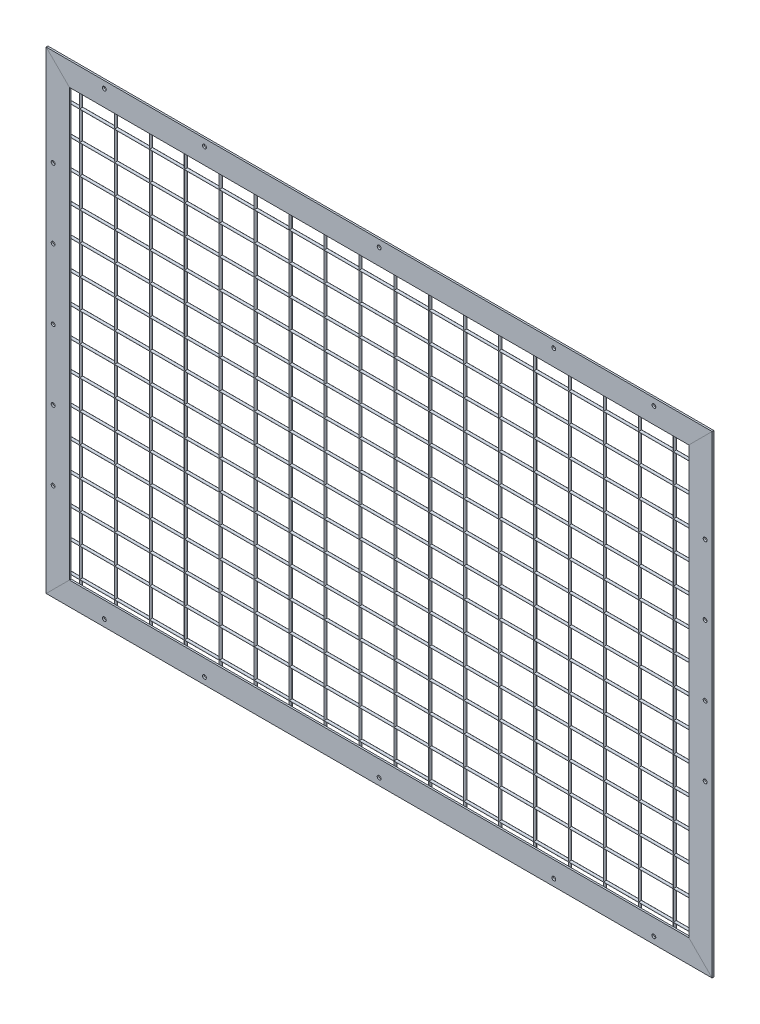
SolidWorks part; units mm, degrees
material "Q235-A GB/T700-2006"
material "Q235-A GB/T700-2006"
material "Q235-A GB/T700-2006"
material "Q235-A GB/T700-2006"
material "Q235-A GB/T700-2006"
material "Q235-A GB/T700-2006"
ref_plane "前视" through (0, 0, 0) normal (0, 0, 1) x (1, 0, 0)
ref_plane "上视" through (0, 0, 0) normal (0, 1, 0) x (1, 0, 0)
ref_plane "右视" through (0, 0, 0) normal (1, 0, 0) x (0, 0, -1)
sketch "草图4" plane through (0, 0, 0) normal (0, 0, 1) x (1, 0, 0)
  line L1 (0, 0) -> (40, 40)
  line L2 (0, 0) -> (0, 813)
  line L3 (0, 813) -> (40, 773)
  line L4 (40, 40) -> (40, 773)
  line L5 (1104, 40) -> (1144, 0)
  line L6 (1104, 40) -> (1104, 773)
  line L7 (1104, 773) -> (1144, 813)
  line L8 (1144, 0) -> (1144, 813)
  dimension "D1" = 813
  dimension "D2" = 45
  dimension "D3" = 1144
  dimension "D4" = 40
  dimension "D5" = 45
  dimension "D6" = 45
  dimension "D7" = 45
extrude "凸台-拉伸2" add sketch "草图4" along normal blind 3
sketch "草图6" plane through (0, 0, 3) normal (0, 0, 1) x (1, 0, 0)
  line L0 (1104, 773) -> (1104, 40) construction
  line L1 (0, 0) -> (1144, 0)
  line L2 (0, 0) -> (40, 40)
  line L3 (40, 40) -> (1104, 40)
  line L4 (1144, 0) -> (1104, 40)
  line L5 (40, 773) -> (0, 813) construction
  line L6 (0, 813) -> (1144, 813)
  line L7 (0, 813) -> (40, 773)
  line L8 (40, 773) -> (1104, 773)
  line L9 (1144, 813) -> (1104, 773)
  line L10 (1144, 0) -> (1144, 813) construction
  line L11 (1144, 813) -> (1104, 773) construction
  line L12 (0, 0) -> (40, 40) construction
extrude "凸台-拉伸3" add sketch "草图6" against normal up to surface (3 mm away) separate body up to face at (20, 406.5, 0)
ref_plane "基准面1" through (0, 25, 0) normal (0, -1, 0) x (-1, 0, 0)
ref_plane "基准面2" through (25, 0, 0) normal (-1, 0, 0) x (0, 0, 1)
sketch "草图7" plane through (0, 25, 0) normal (0, -1, 0) x (-1, 0, 0)
  line L0 (0, 0) -> (-1144, 0) construction
  line L1 (0, -3) -> (0, 0) construction
  circle A0 centre (-55, 2) radius 2
  circle A1 centre (-115, 2) radius 2
  circle A2 centre (-175, 2) radius 2
  circle A3 centre (-235, 2) radius 2
  circle A4 centre (-295, 2) radius 2
  circle A5 centre (-355, 2) radius 2
  circle A6 centre (-415, 2) radius 2
  circle A7 centre (-475, 2) radius 2
  circle A8 centre (-535, 2) radius 2
  circle A9 centre (-595, 2) radius 2
  circle A10 centre (-655, 2) radius 2
  circle A11 centre (-715, 2) radius 2
  circle A12 centre (-775, 2) radius 2
  circle A13 centre (-835, 2) radius 2
  circle A14 centre (-895, 2) radius 2
  circle A15 centre (-955, 2) radius 2
  circle A16 centre (-1015, 2) radius 2
  circle A17 centre (-1075, 2) radius 2
  circle A20 centre (-1195, 2) radius 2 [skipped]
  circle A21 centre (-1135, 2) radius 2 [skipped]
  dimension "D1" = 4
  dimension "D2" = 55
  dimension "D3" = 20
extrude "凸台-拉伸4" add sketch "草图7" against normal offset from surface (763 mm away) 25 separate body up to face at (572, 813, 1.5)
sketch "草图8" plane through (25, 0, 0) normal (-1, 0, 0) x (0, 0, 1)
  line L0 (0, 813) -> (0, 0) construction
  line L2 (-4, 25) -> (0, 25) construction
  circle A0 centre (-2, 47.1) radius 2
  circle A1 centre (-2, 97.1) radius 2
  circle A2 centre (-2, 147.1) radius 2
  circle A3 centre (-2, 197.1) radius 2
  circle A4 centre (-2, 247.1) radius 2
  circle A5 centre (-2, 297.1) radius 2
  circle A6 centre (-2, 347.1) radius 2
  circle A7 centre (-2, 397.1) radius 2
  circle A8 centre (-2, 447.1) radius 2
  circle A9 centre (-2, 497.1) radius 2
  circle A10 centre (-2, 547.1) radius 2
  circle A11 centre (-2, 597.1) radius 2
  circle A12 centre (-2, 647.1) radius 2
  circle A13 centre (-2, 697.1) radius 2
  circle A14 centre (-2, 747.1) radius 2
  dimension "D1" = 4
  dimension "D2" = 22.1
  dimension "D4" = 5
  dimension "D3" = 11
extrude "凸台-拉伸5" add sketch "草图8" against normal offset from surface (1094 mm away) 25 up to face at (1144, 406.5, 1.5)
hole_wizard "M6 间隙孔1" positions "草图10" profile "草图9" hole size "M6" standard "ISO" end condition up to next
sketch "草图10" plane through (0, 0, 3) normal (0, 0, 1) x (1, 0, 0)
  line L0 (0, 406.5) -> (-547.7626, 406.5) construction
  line L1 (0, 813) -> (0, 0) construction
  line L4 (572, 0) -> (572, 801) construction
  line L5 (1144, 813) -> (0, 813) construction
  line L6 (0, 0) -> (1144, 0) construction
  point P0 (100, 801)
  point P2 (572, 801)
  point P12 (12, 646.5)
  point P35 (12, 166.5)
  point P36 (1044, 12)
  point P37 (572, 12)
  point P38 (100, 12)
  point P48 (272, 801)
  point P50 (272, 12)
  point P54 (872, 12)
  point P61 (12, 526.5)
  point P63 (12, 406.5)
  point P65 (12, 286.5)
  point P72 (1132, 526.5)
  point P74 (1132, 406.5)
  point P76 (1132, 286.5)
  point P86 (872, 801)
  point P89 (1044, 801)
  point P91 (1132, 646.5)
  dimension "D1" = 12
  dimension "D2" = 100
  dimension "D3" = 120
  dimension "D4" = 12
  dimension "D5" = 300
  dimension "D7" = 240
sketch "草图9" plane through (100, 801, 3) normal (1, 0, 0) x (0, -1, 0)
  line L0 (0, 0) -> (0, 3.001)
  line L1 (0, 3.001) -> (3.3, 3.001)
  line L2 (3.3, 3.001) -> (3.3, 0)
  line L5 (3.3, 0) -> (0, 0)
  line L11 (0, -6.35) -> (0, 107.95) construction
  dimension "通孔孔直径" = 6.6
  dimension "通孔孔深度" = 3.001
sketch "草图11" plane through (0, 0, 3) normal (0, 0, 1) x (1, 0, 0)
  line L1 (1144, 0) -> (1061, 0)
  line L2 (1144, 0) -> (1144, 158)
  line L3 (1144, 158) -> (1061, 158)
  line L4 (1061, 0) -> (1061, 158)
  dimension "D1" = 83
  dimension "D2" = 158
extrude "切除-拉伸1" [suppressed] cut sketch "草图11" against normal blind 10
sketch "草图14" plane through (0, 0, 3) normal (0, 0, 1) x (1, 0, 0)
  line L0 (1144, 813) -> (0, 813) construction
  line L1 (1144, 0) -> (1104, 0)
  line L2 (1144, 0) -> (1144, 813)
  line L3 (1144, 813) -> (1104, 813)
  line L4 (1104, 0) -> (1104, 813)
  dimension "D1" = 40
extrude "切除-拉伸4" [suppressed] cut sketch "草图14" against normal blind 433
